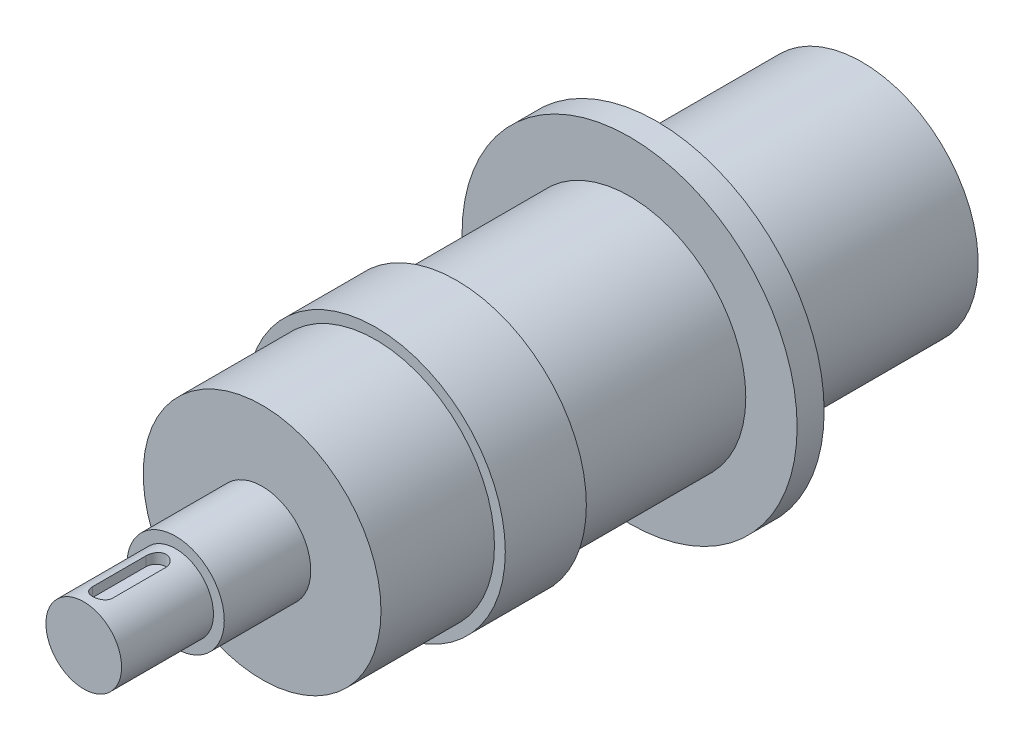
SolidWorks part; units mm, degrees
ref_plane "Front Plane" through (0, 0, 0) normal (0, 0, 1) x (1, 0, 0)
ref_plane "Top Plane" through (0, 0, 0) normal (0, 1, 0) x (1, 0, 0)
ref_plane "Right Plane" through (0, 0, 0) normal (1, 0, 0) x (0, 0, -1)
other "Configuration Table"
sketch "Sketch1" plane through (0, 0, 38) normal (0, 0, 1) x (1, 0, 0)
  circle A0 centre (0, 0) radius 21.5
  dimension "D1" = 43
extrude "Boss-Extrude1" add sketch "Sketch1" along normal blind 37 contours A0
sketch "Sketch2" plane through (0, 0, 75) normal (0, 0, 1) x (1, 0, 0)
  circle A0 centre (0, 0) radius 24
  dimension "D1" = 48
extrude "Boss-Extrude2" add sketch "Sketch2" along normal blind 15
sketch "Sketch3" plane through (0, 0, 90) normal (0, 0, 1) x (1, 0, 0)
  circle A0 centre (0, 0) radius 22
  dimension "D1" = 44
extrude "Boss-Extrude3" add sketch "Sketch3" along normal blind 21 contours A0
sketch "Sketch4" plane through (0, 0, 111) normal (0, 0, 1) x (1, 0, 0)
  circle A0 centre (0, 0) radius 9
  dimension "D1" = 18
extrude "Boss-Extrude4" add sketch "Sketch4" along normal blind 16
sketch "Sketch5" plane through (0, 0, 127) normal (0, 0, 1) x (1, 0, 0)
  circle A0 centre (0, 0) radius 7
  dimension "D1" = 14
extrude "Boss-Extrude5" add sketch "Sketch5" along normal blind 17 contours A0
sketch "Sketch6" plane through (0, 0, 0) normal (0, 1, 0) x (1, 0, 0)
  line L0 (0, -130.6399) -> (0, -140.5) construction
  line L1 (1.85, -130.6399) -> (1.85, -140.5)
  line L2 (-1.85, -130.6399) -> (-1.85, -140.5)
  line L3 (-7, -144) -> (7, -144) construction
  arc A0 (1.85, -130.6399) -> (-1.85, -130.6399) centre (0, -130.6399) ccw
  arc A1 (-1.85, -140.5) -> (1.85, -140.5) centre (0, -140.5) ccw
  point P3 (0, -135.57)
  dimension "D1" = 1.85
  dimension "D2" = 13.3601
  dimension "D3" = 3.5
extrude "Cut-Extrude1" cut sketch "Sketch6" against normal blind 25 from offset 30
sketch "Sketch7" plane through (0, 0, 38) normal (0, 0, -1) x (-1, 0, 0)
  circle A0 centre (0, 0) radius 21.5
  dimension "D1" = 43
extrude "Boss-Extrude6" add sketch "Sketch7" along normal blind 38
sketch "Sketch9" plane through (0, 0, 38) normal (0, 0, 1) x (1, 0, 0)
  circle A0 centre (0, 0) radius 31
  dimension "D1" = 62
extrude "Boss-Extrude7" add sketch "Sketch9" along normal blind 5
sketch "Sketch12" plane through (0, 0, 0) normal (0, 0, -1) x (-1, 0, 0)
  point P0 (0, 0)
hole_wizard "M8 Tapped Hole1" positions "3DSketch3" profile "Sketch13" tap size "M8" standard "GB"
sketch3d "3DSketch3"
  point P0 (0, 0, 0)
  point P4 (0, 0, 0)
  point P6 (0, 0, 0)
  point P10 (0, 0, 0)
sketch "Sketch13" plane through (0, 0, 0) normal (1, 0, 0) x (0, 1, 0)
  line L0 (0, 0) -> (0, 37.0429)
  line L1 (0, 37.0429) -> (3.4, 35)
  line L2 (3.4, 35) -> (3.4, 0)
  line L5 (3.4, 0) -> (0, 0)
  line L10 (0, 37.0429) -> (-3.4, 35) construction
  line L11 (0, -6.35) -> (0, 107.95) construction
  dimension "螺纹孔钻头直径" = 6.8
  dimension "螺纹孔钻头深度" = 35
  dimension "导头角度" = 118
cosmetic thread "Cosmetic thread 5" parameters "D1"=16, "D2"=8
cosmetic thread "Cosmetic thread 6" parameters "D1"=16, "D2"=8
cosmetic thread "Cosmetic thread 7" parameters "D1"=16, "D2"=8
cosmetic thread "Cosmetic thread 8" parameters "D1"=16, "D2"=8
